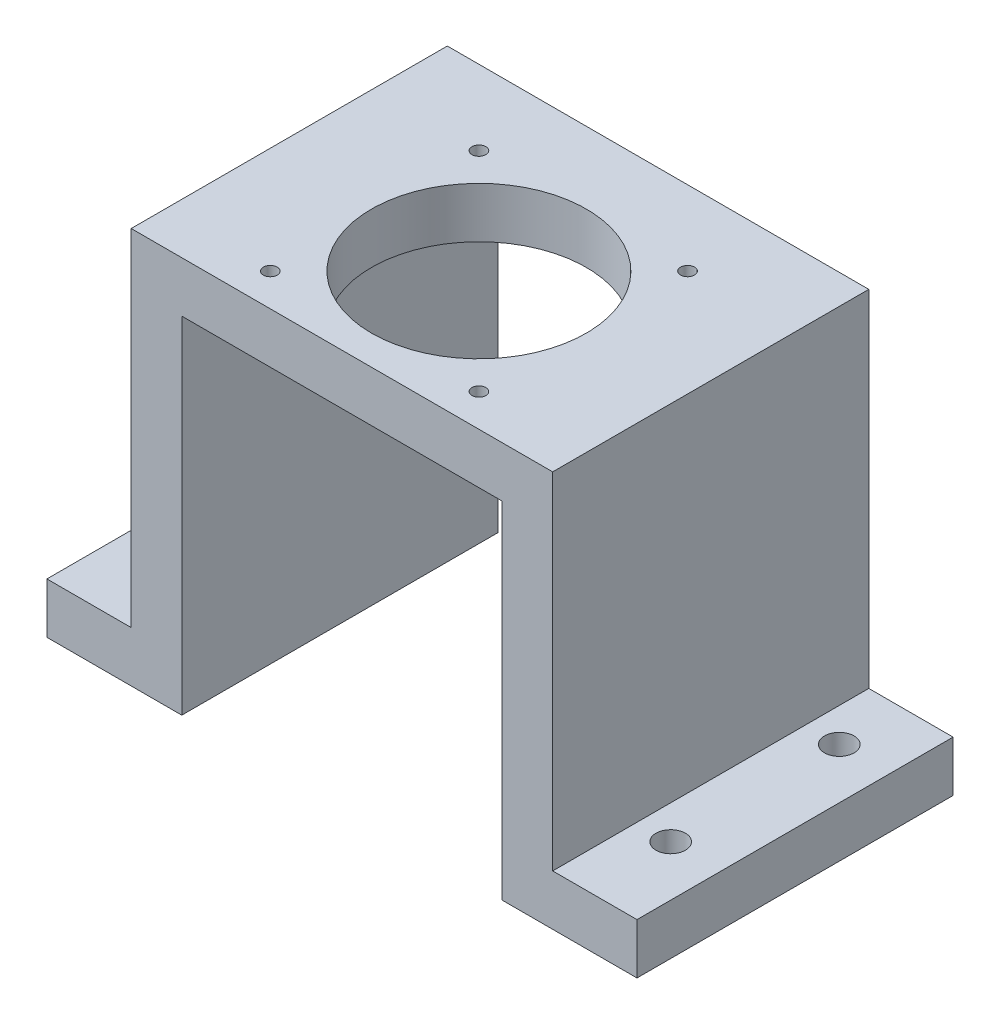
from build123d import *

# Parameters (mm, degrees)
EXTRUDE_THIN1_DEPTH = 75
SKETCH2_R           = 25.5
CUT_EXTRUDE1_DEPTH  = 140.143810498
SKETCH4_R           = 3.5
CUT_EXTRUDE3_DEPTH  = 132.335448376
M4_TAPPED_HOLE1_D   = 3.3


with BuildPart() as part:
    # Sketch1 → Extrude-Thin1 (new body)
    with BuildSketch(Plane.XY):
        Polygon((-70, 0), (-50, 0), (-50, 82), (50, 82), (50, 0), (70, 0), (70, -12), (38, -12), (38, 70), (-38, 70), (-38, -12), (-70, -12), align=None)
    extrude(amount=EXTRUDE_THIN1_DEPTH)

    # Sketch2 → Cut-Extrude1 (cut, through all)
    with BuildSketch(Plane(origin=(0, 82, 0), x_dir=(1, 0, 0), z_dir=(0, 1, 0))):
        with Locations(Location((0, -42.5, 0), (0, 0, 270))):
            Circle(SKETCH2_R)
    extrude(amount=-CUT_EXTRUDE1_DEPTH, mode=Mode.SUBTRACT)

    # Sketch4 → Cut-Extrude3 (cut, through all)
    with BuildSketch(Plane(origin=(0, 0, 0), x_dir=(1, 0, 0), z_dir=(0, 1, 0))):
        with Locations(Location((-58, -15, 0), (0, 0, 270))):
            Circle(SKETCH4_R)
        with Locations(Location((58, -15, 0), (0, 0, 90))):
            Circle(SKETCH4_R)
        with Locations(Location((58, -55, 0), (0, 0, 270))):
            Circle(SKETCH4_R)
        with Locations(Location((-58, -55, 0), (0, 0, 90))):
            Circle(SKETCH4_R)
    extrude(amount=-CUT_EXTRUDE3_DEPTH, mode=Mode.SUBTRACT)

    # M4 Tapped Hole1 (through all)
    with Locations(Plane(origin=(0, 82, 0), x_dir=(1, 0, 0), z_dir=(0, 1, 0))):
        with Locations((-24.748737342, -17.751262658), (24.748737342, -17.751262658), (24.748737342, -67.248737342), (-24.748737342, -67.248737342)):
            Hole(M4_TAPPED_HOLE1_D / 2)


solid = part.part
